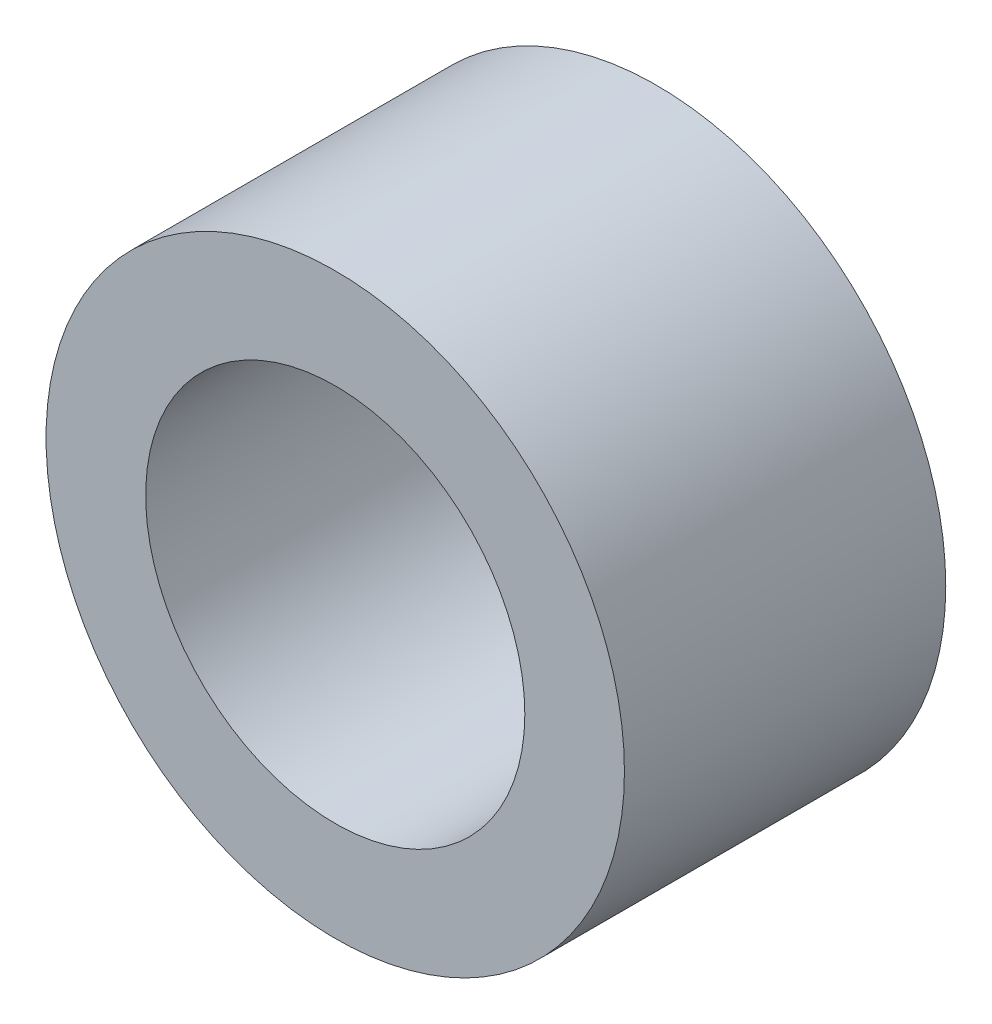
from build123d import *

# Parameters (mm, degrees)
SKETCH1_R           = 22.5
SKETCH1_R_2         = 14.75
BOSS_EXTRUDE1_DEPTH = 25


with BuildPart() as part:
    # Sketch1 → Boss-Extrude1 (new body)
    with BuildSketch(Plane.XY):
        Circle(SKETCH1_R)
        Circle(SKETCH1_R_2, mode=Mode.SUBTRACT)
    extrude(amount=BOSS_EXTRUDE1_DEPTH)


solid = part.part
